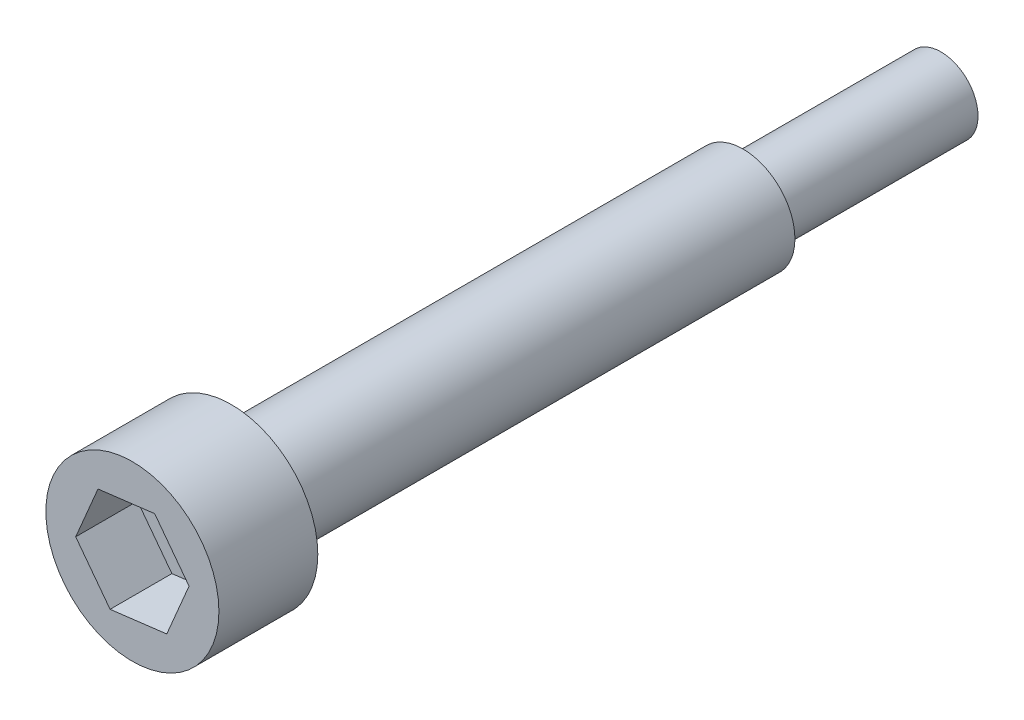
SolidWorks part; units mm, degrees
ref_plane "前视基准面" through (0, 0, 0) normal (0, 0, 1) x (1, 0, 0)
ref_plane "上视基准面" through (0, 0, 0) normal (0, 1, 0) x (1, 0, 0)
ref_plane "右视基准面" through (0, 0, 0) normal (1, 0, 0) x (0, 0, -1)
sketch "草图1" plane through (0, 0, 0) normal (0, 0, 1) x (1, 0, 0)
  circle A0 centre (-26.1593, -76.9973) radius 7
  dimension "D1" = 14
extrude "凸台-拉伸1" add sketch "草图1" along normal blind 8
sketch "草图2" plane through (0, 0, 0) normal (0, 0, -1) x (-1, 0, 0)
  circle A0 centre (26.1593, -76.9973) radius 4.191 construction
  circle A1 centre (26.1593, -76.9973) radius 4.191
extrude "凸台-拉伸2" add sketch "草图2" along normal up to surface (41.4 mm away)
sketch "草图3" plane through (0, 0, -41.4) normal (0, 0, -1) x (-1, 0, 0)
  circle A0 centre (26.1593, -76.9973) radius 3
  dimension "D1" = 6
extrude "凸台-拉伸3" add sketch "草图3" along normal up to surface (16 mm away)
sketch "草图4" plane through (0, 0, 8) normal (0, 0, 1) x (1, 0, 0)
  line L1 (-24.3561, -72.745) -> (-28.9403, -73.3096)
  line L2 (-28.9403, -73.3096) -> (-30.7434, -77.5619)
  line L3 (-30.7434, -77.5619) -> (-27.9624, -81.2496)
  line L4 (-27.9624, -81.2496) -> (-23.3782, -80.685)
  line L5 (-23.3782, -80.685) -> (-21.5751, -76.4327)
  line L6 (-21.5751, -76.4327) -> (-24.3561, -72.745)
  circle A0 centre (-26.1593, -76.9973) radius 4 construction
  dimension "D1" = 8
extrude "切除-拉伸1" cut sketch "草图4" against normal blind 5
